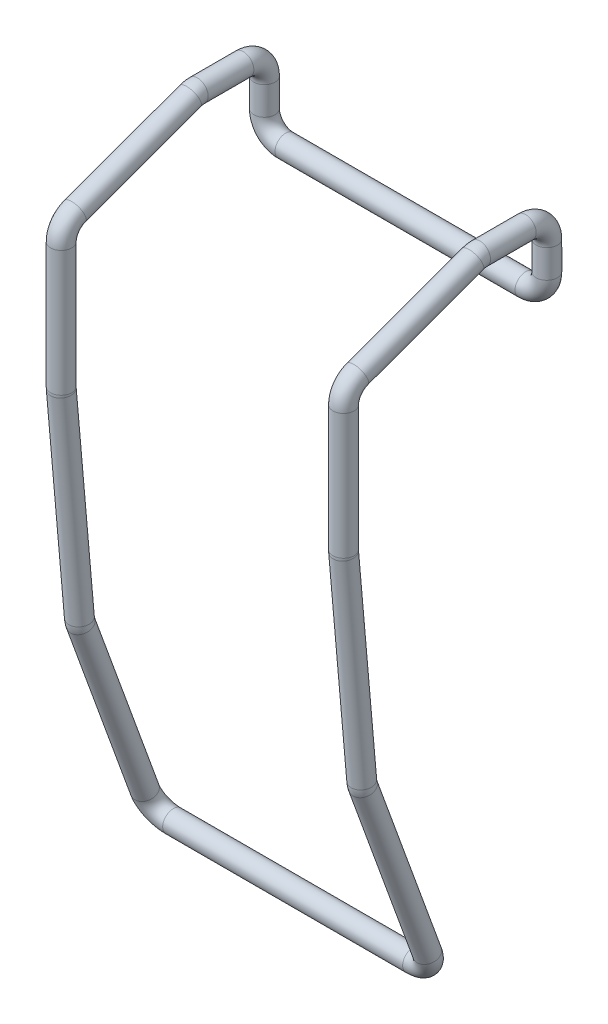
SolidWorks part; units mm, degrees
material "AISI 304"
ref_plane "Front Plane" through (0, 0, 0) normal (0, 0, 1) x (1, 0, 0)
ref_plane "Top Plane" through (0, 0, 0) normal (0, 1, 0) x (1, 0, 0)
ref_plane "Right Plane" through (0, 0, 0) normal (1, 0, 0) x (0, 0, -1)
sketch "Sketch1" plane through (0, 0, 0) normal (1, 0, 0) x (0, 0, -1)
  circle A0 centre (0, 0) radius 1.5
  dimension "D1" = 3
sketch3d "3DSketch1"
  line L0 (0, 0, 0) -> (17, 0, 0)
  line L1 (20, 2.8191, 1.0261) -> (20, 27.8196, 10.1255)
  line L2 (20, 0, 0) -> (20, 0, 6.8541) construction
  line L3 (20, 28.5842, 10.295) -> (20, 57.9461, 12.8639)
  line L4 (20, 28.1908, 10.2606) -> (-43.3011, 28.1908, 10.2606) construction
  line L5 (20, 58.2076, 12.8753) -> (20, 75.976, 12.8753)
  line L6 (20, 78.7951, 10.9013) -> (20, 84.7361, -5.4215)
  line L7 (20, 78.0766, 12.8753) -> (88.4487, 78.0766, 12.8753) construction
  line L8 (20, 84.917, -6.4476) -> (20, 84.917, -12.9186)
  line L9 (20, 81.917, -15.9186) -> (20, 77.917, -15.9186)
  line L10 (17, 74.917, -15.9186) -> (0, 74.917, -15.9186)
  arc A0 (17, 74.917, -15.9186) -> (20, 77.917, -15.9186) centre (17, 77.917, -15.9186) ccw
  arc A1 (20, 81.917, -15.9186) -> (20, 84.917, -12.9186) centre (20, 81.917, -12.9186) ccw
  arc A2 (20, 84.917, -6.4476) -> (20, 84.7361, -5.4215) centre (20, 81.917, -6.4476) ccw
  arc A3 (20, 75.976, 12.8753) -> (20, 78.7951, 10.9013) centre (20, 75.976, 9.8753) ccw
  arc A4 (20, 58.2076, 12.8753) -> (20, 57.9461, 12.8639) centre (20, 58.2076, 9.8753) ccw
  arc A5 (20, 28.5842, 10.295) -> (20, 27.8196, 10.1255) centre (20, 28.8457, 7.3064) ccw
  arc A6 (20, 2.8191, 1.0261) -> (17, 0, 0) centre (17, 2.8191, 1.0261) ccw
  point P15 (20, 74.917, -15.9186)
  point P16 (17, 77.917, -12.9186)
  point P19 (20, 84.917, -15.9186)
  point P20 (23, 81.917, -12.9186)
  point P23 (20, 84.917, -5.9186)
  point P24 (23, 81.917, -6.4476)
  point P27 (20, 78.0766, 12.8753)
  point P29 (17, 75.976, 9.8753)
  point P32 (20, 58.0766, 12.8753)
  point P33 (23, 58.2076, 9.8753)
  point P36 (20, 28.1908, 10.2606)
  point P38 (23, 28.8457, 7.3064)
  point P41 (20, 0, 0)
  point P43 (17, 3.8451, -1.793)
  dimension "D13" = 3
  dimension "D1" = 20
  dimension "D2" = 90
  dimension "D3" = 70
  dimension "D4" = 30
  dimension "D5" = 165
  dimension "D6" = 30
  dimension "D7" = 90
  dimension "D8" = 20
  dimension "D9" = 90
  dimension "D10" = 20
  dimension "D11" = 10
  dimension "D12" = 10
sweep "Sweep1" add profiles "Sketch1" path "3DSketch1"
mirror "Mirror1" about plane through (0, 74.917, -15.9186) normal (-1, 0, 0) of "Sweep1"
